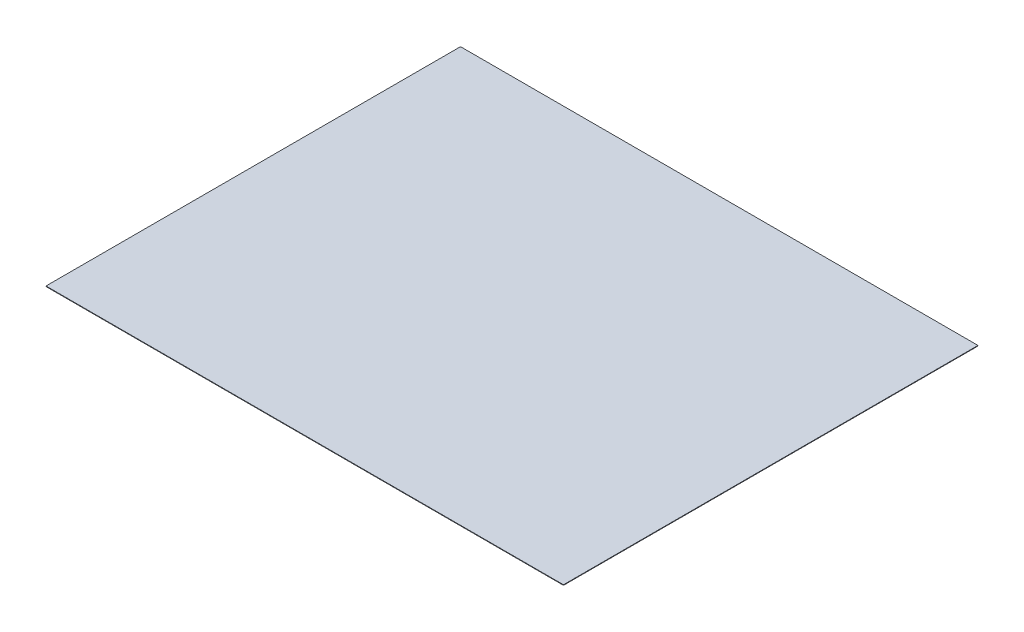
SolidWorks part; units mm, degrees
ref_plane "Front Plane" through (0, 0, 0) normal (0, 0, 1) x (1, 0, 0)
ref_plane "Top Plane" through (0, 0, 0) normal (0, 1, 0) x (1, 0, 0)
ref_plane "Right Plane" through (0, 0, 0) normal (1, 0, 0) x (0, 0, -1)
sketch "Sketch1" plane through (0, 0, 0) normal (0, 1, 0) x (1, 0, 0)
  line L1 (-500, -400.5) -> (500, -400.5)
  line L2 (-500, -400.5) -> (-500, 400.5)
  line L3 (-500, 400.5) -> (500, 400.5)
  line L4 (500, -400.5) -> (500, 400.5)
  line L5 (-500, -400.5) -> (500, 400.5) construction
  line L6 (-500, 400.5) -> (500, -400.5) construction
  point P0 (0, 0)
  dimension "D1" = 1000
  dimension "D2" = 801
extrude "Boss-Extrude1" add sketch "Sketch1" along normal blind 1
